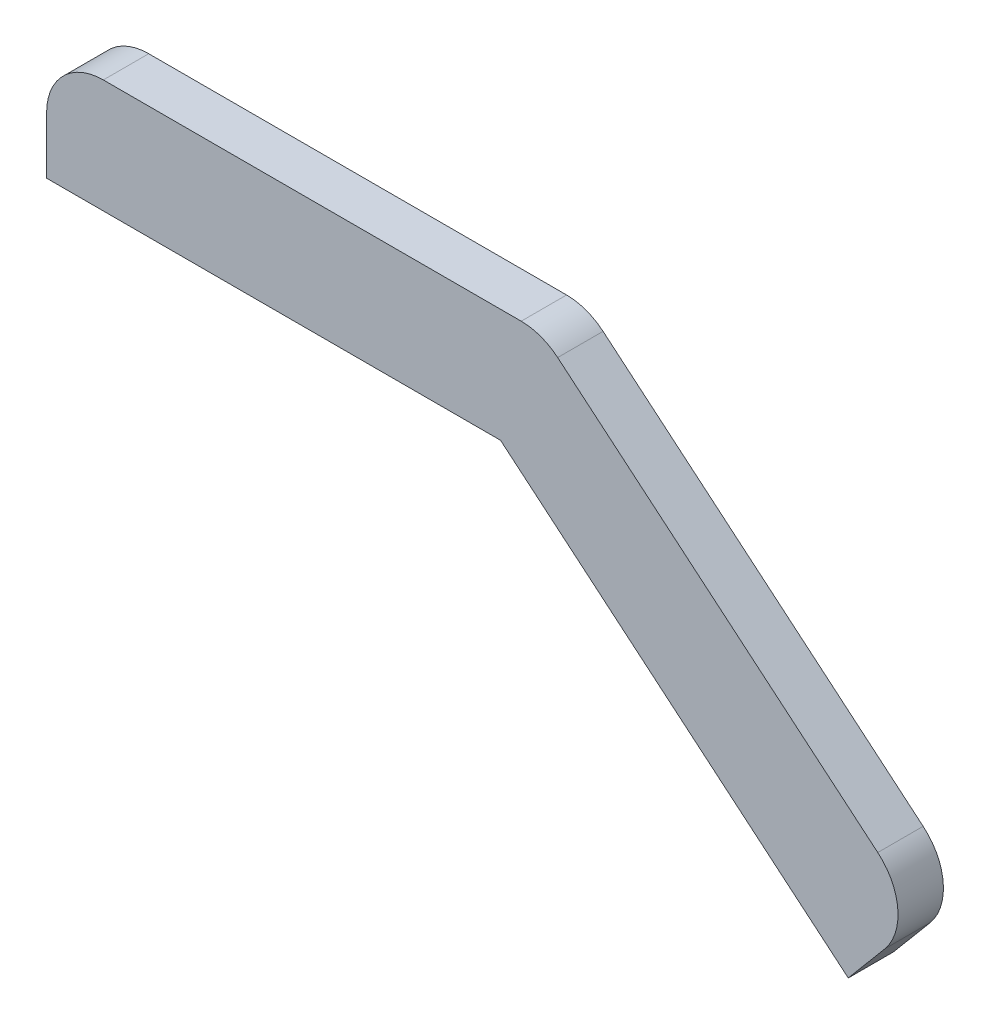
from build123d import *

# Parameters (mm, degrees)
BOSS_EXTRUDE1_DEPTH = 8
FILLET1_R           = 10


with BuildPart() as part:
    # Sketch1 → Boss-Extrude1 (new body)
    with BuildSketch(Plane.XY):
        Polygon((0, 0), (80, 0), (141.28355545, -51.423008775), (154.139307643, -36.102119913), (87.279404685, 20), (0, 20), align=None)
    extrude(amount=BOSS_EXTRUDE1_DEPTH)

    # Fillet1
    fillet1_edges = [part.edges().sort_by_distance(p)[0] for p in [
        (0, 20, 4),
        (87.279404685, 20, 4),
        (154.139307643, -36.102119913, 4),
    ]]
    fillet(fillet1_edges, radius=FILLET1_R)


solid = part.part
